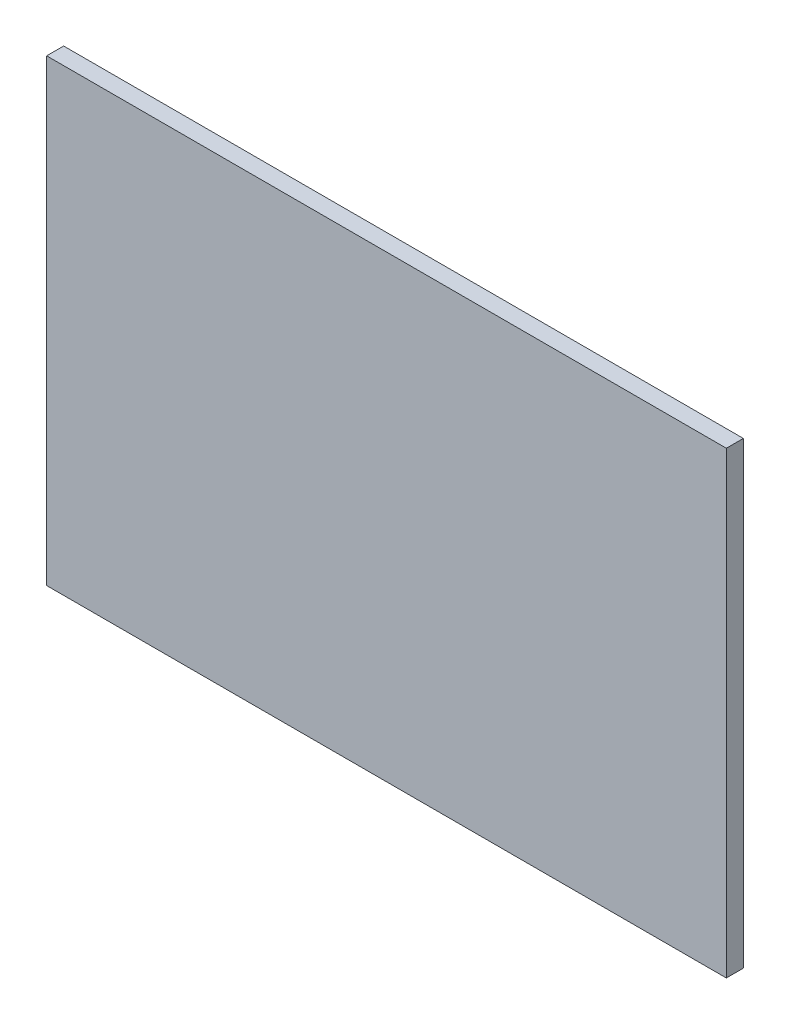
from build123d import *

# Parameters (mm, degrees)
SKETCH1_W           = 400
SKETCH1_H           = 270
BOSS_EXTRUDE1_DEPTH = 5


with BuildPart() as part:
    # Sketch1 → Boss-Extrude1 (new, symmetric)
    with BuildSketch(Plane.XY):
        Rectangle(SKETCH1_W, SKETCH1_H)
    extrude(amount=BOSS_EXTRUDE1_DEPTH, both=True)


solid = part.part
